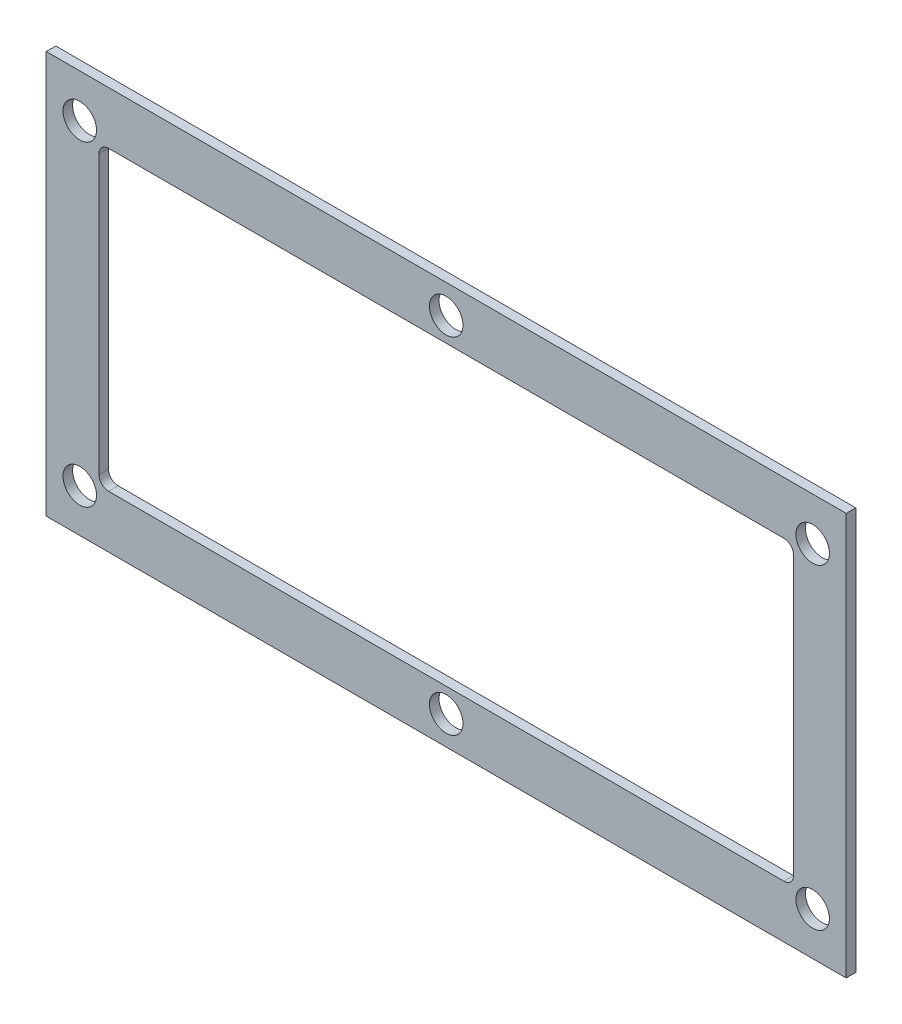
from build123d import *

# Parameters (mm, degrees)
SKETCH1_W           = 83.5
SKETCH1_H           = 42
SKETCH1_R           = 1.75
SKETCH1_W_2         = 72.5
SKETCH1_H_2         = 31
BOSS_EXTRUDE1_DEPTH = 1
FILLET1_R           = 1


with BuildPart() as part:
    # Sketch1 → Boss-Extrude1 (new body)
    with BuildSketch(Plane.XY):
        Rectangle(SKETCH1_W, SKETCH1_H)
        with Locations((-38.25, 16.5)):
            Circle(SKETCH1_R, mode=Mode.SUBTRACT)
        with Locations((38.25, 16.5)):
            Circle(SKETCH1_R, mode=Mode.SUBTRACT)
        with Locations((38.25, -16.5)):
            Circle(SKETCH1_R, mode=Mode.SUBTRACT)
        with Locations((-38.25, -16.5)):
            Circle(SKETCH1_R, mode=Mode.SUBTRACT)
        with Locations((0, 18)):
            Circle(SKETCH1_R, mode=Mode.SUBTRACT)
        with Locations((0, -18)):
            Circle(SKETCH1_R, mode=Mode.SUBTRACT)
        Rectangle(SKETCH1_W_2, SKETCH1_H_2, mode=Mode.SUBTRACT)
    extrude(amount=BOSS_EXTRUDE1_DEPTH)

    # Fillet1
    fillet1_edges = [part.edges().sort_by_distance(p)[0] for p in [
        (-36.25, 15.5, 0.5),
        (-36.25, -15.5, 0.5),
        (36.25, -15.5, 0.5),
        (36.25, 15.5, 0.5),
    ]]
    fillet(fillet1_edges, radius=FILLET1_R)


solid = part.part
